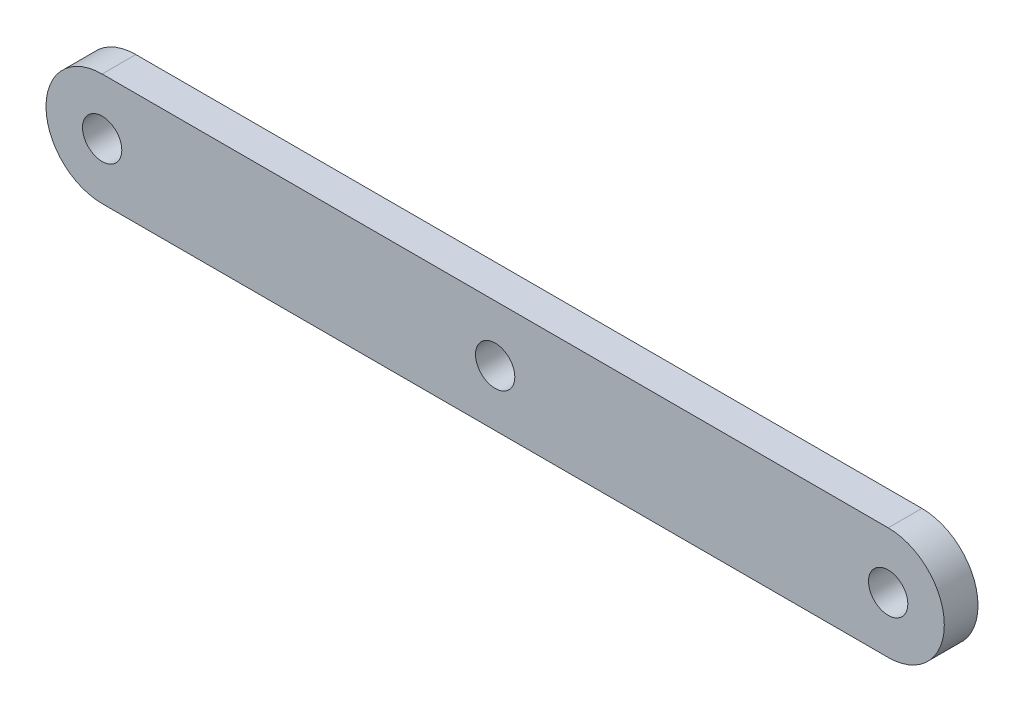
from build123d import *

# Parameters (mm, degrees)
BOSS_EXTRUDE1_DEPTH = 6
SKETCH2_R           = 3.5
CUT_EXTRUDE1_DEPTH  = 95
SKETCH3_R           = 3.5
CUT_EXTRUDE2_DEPTH  = 10


with BuildPart() as part:
    # Sketch1 → Boss-Extrude1 (new body)
    with BuildSketch(Plane.XY):
        with BuildLine():
            Line((0, 10), (140, 10))
            ThreePointArc((140, 10), (150, 0), (140, -10))
            Line((140, -10), (0, -10))
            ThreePointArc((0, -10), (-10, 0), (0, 10))
        make_face()
    extrude(amount=BOSS_EXTRUDE1_DEPTH)

    # Sketch2 → Cut-Extrude1 (cut)
    with BuildSketch(Plane.XY.offset(6)):
        Circle(SKETCH2_R)
        with Locations((140, 0)):
            Circle(SKETCH2_R)
    extrude(amount=-CUT_EXTRUDE1_DEPTH, mode=Mode.SUBTRACT)

    # Sketch3 → Cut-Extrude2 (cut)
    with BuildSketch(Plane.XY.offset(6)):
        with Locations((70, 0)):
            Circle(SKETCH3_R)
    extrude(amount=-CUT_EXTRUDE2_DEPTH, mode=Mode.SUBTRACT)


solid = part.part
